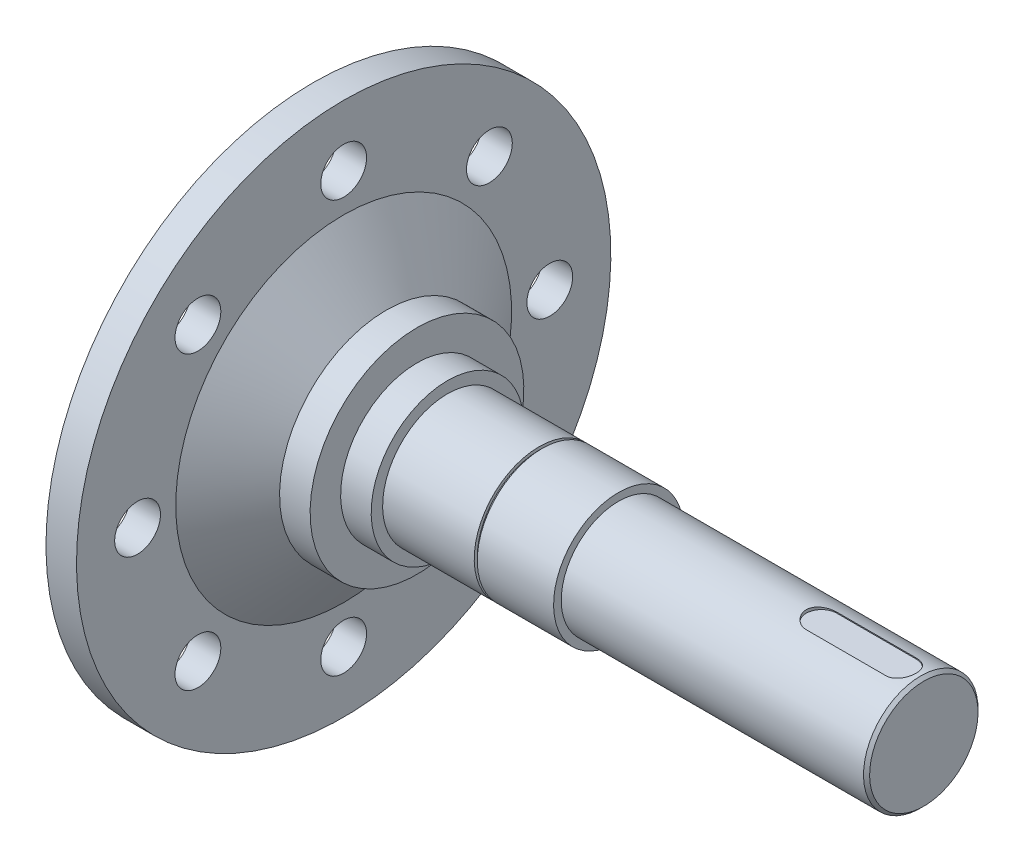
SolidWorks part; units mm, degrees
ref_plane "前视基准面" through (0, 0, 0) normal (0, 0, 1) x (1, 0, 0)
ref_plane "上视基准面" through (0, 0, 0) normal (0, 1, 0) x (1, 0, 0)
ref_plane "右视基准面" through (0, 0, 0) normal (1, 0, 0) x (0, 0, -1)
other "Configuration Table"
sketch "草图1" plane through (0, 0, 0) normal (0, 0, 1) x (1, 0, 0)
  line L0 (0, 0) -> (0, 175)
  line L1 (0, 175) -> (20, 175)
  line L2 (20, 175) -> (20, 110)
  line L3 (20, 110) -> (48.0083, 70)
  line L4 (48.0083, 70) -> (68.0083, 70)
  line L5 (68.0083, 70) -> (68.0083, 50)
  line L6 (68.0083, 50) -> (88.0083, 50)
  line L7 (88.0083, 50) -> (88.0083, 42.5)
  line L8 (88.0083, 42.5) -> (148, 42.5)
  line L9 (148, 42.5) -> (148, 40.5)
  line L10 (148, 40.5) -> (150, 40.5)
  line L11 (150, 40.5) -> (150, 42.5)
  line L12 (150, 42.5) -> (200, 42.5)
  line L13 (200, 42.5) -> (200, 37.5)
  line L14 (200, 37.5) -> (400, 37.5)
  line L15 (400, 37.5) -> (400, 0)
  line L16 (400, 0) -> (0, 0)
  point P23 (58.0083, 70)
  dimension "D1" = 175
  dimension "D2" = 150
  dimension "D3" = 400
  dimension "D4" = 20
  dimension "D5" = 110
  dimension "D6" = 145
  dimension "D7" = 70
  dimension "D8" = 20
  dimension "D9" = 50
  dimension "D10" = 42.5
  dimension "D11" = 20
  dimension "D12" = 50
  dimension "D13" = 2
  dimension "D14" = 2
  dimension "D15" = 37.5
revolve "旋转1" add sketch "草图1" angle 360 about L16
sketch "草图2" plane through (0, 0, 0) normal (-1, 0, 0) x (0, 0, 1)
  circle A0 centre (0, 0) radius 45
  dimension "D1" = 90
extrude "切除-拉伸1" cut sketch "草图2" against normal blind 30 contours A0
chamfer "倒角1" distance 10 angle 45 1 edges at (0, -45, 0)
ref_plane "基准面1" through (0, 37.5, 0) normal (0, 1, 0) x (1, 0, 0)
sketch "草图3" plane through (0, 37.5, 0) normal (0, 1, 0) x (1, 0, 0)
  line L0 (333, 0) -> (385, 0) construction
  line L1 (333, 10) -> (385, 10)
  line L2 (333, -10) -> (385, -10)
  line L3 (400, -37.5) -> (400, 37.5) construction
  arc A0 (333, 10) -> (333, -10) centre (333, 0) ccw
  arc A1 (385, -10) -> (385, 10) centre (385, 0) ccw
  point P2 (359, 0)
  dimension "D2" = 10
  dimension "D1" = 52
  dimension "D3" = 15
extrude "切除-拉伸2" cut sketch "草图3" against normal blind 2
chamfer "倒角2" distance 2 angle 45 1 edges at (400, 37.5, 0)
sketch "草图4" plane through (0, 0, 0) normal (-1, 0, 0) x (0, 0, 1)
  circle A0 centre (0, 0) radius 135 construction
  circle A1 centre (0, 135) radius 15
  circle A2 centre (95.4594, 95.4594) radius 15
  circle A3 centre (135, 0) radius 15
  circle A4 centre (95.4594, -95.4594) radius 15
  circle A5 centre (0, -135) radius 15
  circle A6 centre (-95.4594, -95.4594) radius 15
  circle A7 centre (-135, 0) radius 15
  circle A8 centre (-95.4594, 95.4594) radius 15
  dimension "D1" = 270
  dimension "D2" = 30
  dimension "D3" = 8
extrude "切除-拉伸3" cut sketch "草图4" against normal blind 50
